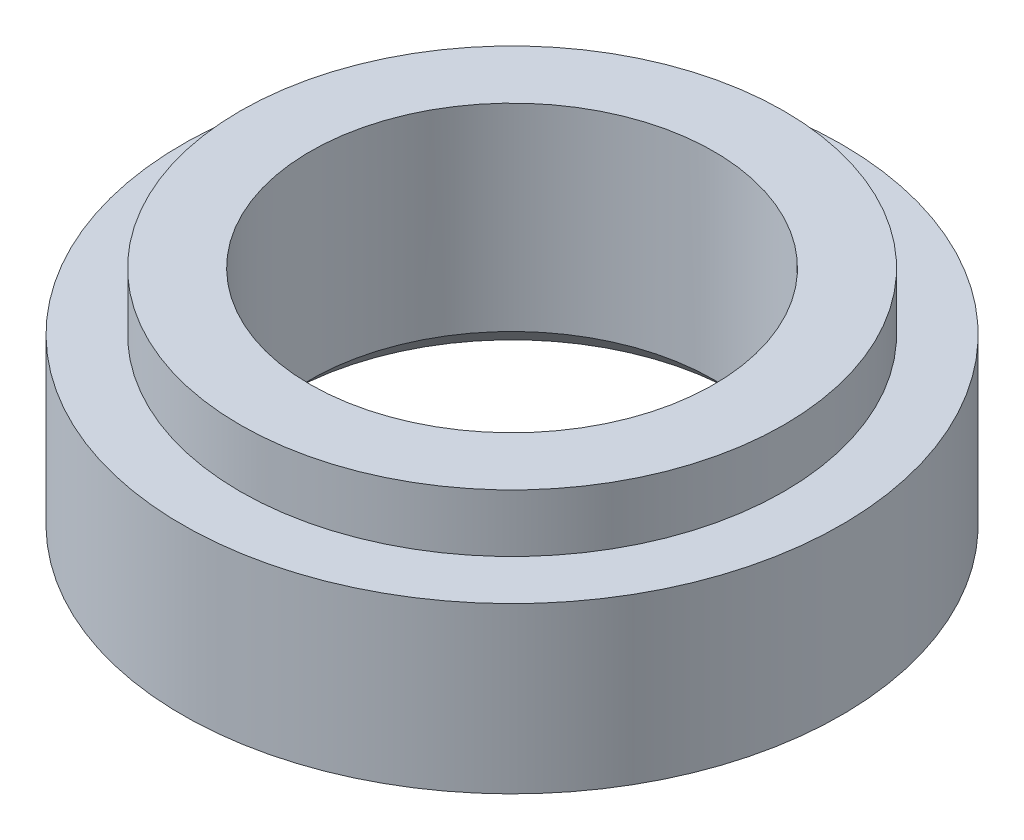
SolidWorks part; units mm, degrees
material "35#"
ref_plane "Front Plane" through (0, 0, 0) normal (0, 0, 1) x (1, 0, 0)
ref_plane "Top Plane" through (0, 0, 0) normal (0, 1, 0) x (1, 0, 0)
ref_plane "Right Plane" through (0, 0, 0) normal (1, 0, 0) x (0, 0, -1)
sketch "Sketch1" plane through (0, 0, 0) normal (0, 0, 1) x (1, 0, 0)
  line L0 (0, 0) -> (20, 0)
  line L1 (20, 0) -> (20, 10)
  line L2 (20, 10) -> (16.5, 10)
  line L3 (16.5, 10) -> (16.5, 13.5)
  line L4 (16.5, 13.5) -> (0, 13.5)
  line L5 (0, 0) -> (0, 13.5) construction
  line L6 (0, 0) -> (0, 13.5)
  dimension "D1" = 10
  dimension "D2" = 3.5
  dimension "D3" = 40
  dimension "D4" = 33
revolve "Revolve1" add sketch "Sketch1" angle 360 about L5
hole_wizard "G3/4 Tapped Hole1" positions "Sketch2" profile "Sketch3" tap size "G3/4" standard "GB"
sketch "Sketch2" plane through (0, 13.5, 0) normal (0, 1, 0) x (1, 0, 0)
  point P0 (0, 0)
sketch "Sketch3" plane through (0, 13.5, 0) normal (1, 0, 0) x (0, 0, 1)
  line L0 (0, 0) -> (0, 65.6805)
  line L1 (0, 65.6805) -> (12.25, 58.32)
  line L2 (12.25, 58.32) -> (12.25, 0)
  line L5 (12.25, 0) -> (0, 0)
  line L10 (0, 65.6805) -> (-12.25, 58.32) construction
  line L11 (0, -6.35) -> (0, 107.95) construction
  dimension "螺纹孔钻头直径" = 24.5
  dimension "螺纹孔钻头深度" = 58.32
  dimension "导头角度" = 118
cosmetic thread "Cosmetic thread 1" parameters "D1"=52.88, "D2"=26.441
chamfer "Chamfer1" distance 1.5 angle 45 1 edges at (0, 0, -12.25)
